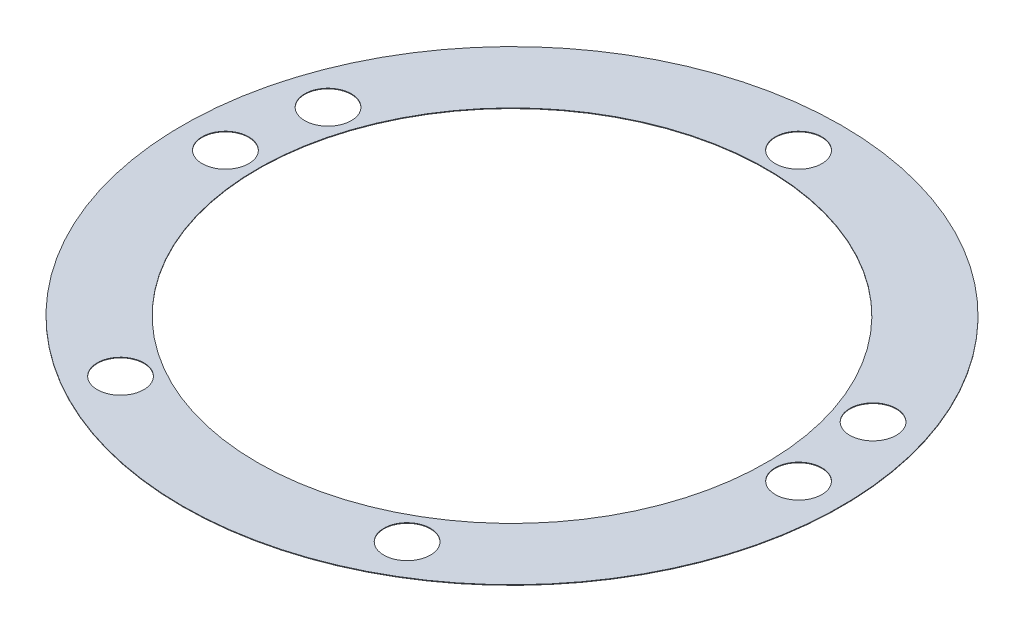
from build123d import *

# Parameters (mm, degrees)
SKETCH1_R                       = 146.05
SKETCH1_R_2                     = 112.776
BOSS_EXTRUDE1_DEPTH             = 0.254
F_13_16_0_8125_DIAMETER_HOLE1_D = 20.6375
F_13_16_0_8125_DIAMETER_HOLE2_D = 20.6375


with BuildPart() as part:
    # Sketch1 → Boss-Extrude1 (new body)
    with BuildSketch(Plane(origin=(0, 0, 0), x_dir=(1, 0, 0), z_dir=(0, 1, 0))):
        with Locations(Location((0, 0, 0), (0, 0, 270))):
            Circle(SKETCH1_R)
        with Locations(Location((0, 0, 0), (0, 0, 270))):
            Circle(SKETCH1_R_2, mode=Mode.SUBTRACT)
    extrude(amount=BOSS_EXTRUDE1_DEPTH)

    # 13/16 (0.8125) Diameter Hole1 (through all)
    with Locations(Plane(origin=(0, 0.254, 0), x_dir=(1, 0, 0), z_dir=(0, 1, 0))):
        with Locations((0, 127)):
            Hole(F_13_16_0_8125_DIAMETER_HOLE1_D / 2)

    # 13/16 (0.8125) Diameter Hole2 (through all)
    with Locations(Plane(origin=(0, 0, 0), x_dir=(-1, 0, 0), z_dir=(0, -1, 0))):
        with Locations((-63.5, -109.982), (-120.77, 39.243), (-127, 0)):
            f_13_16_0_8125_diameter_hole2 = Hole(F_13_16_0_8125_DIAMETER_HOLE2_D / 2)

    # Mirror1: 13/16 (0.8125) Diameter Hole2 across plane
    add(f_13_16_0_8125_diameter_hole2.mirror(Plane(origin=(0, 0, 0), x_dir=(0, 0, 1), z_dir=(1, 0, 0))), mode=Mode.SUBTRACT)


solid = part.part
